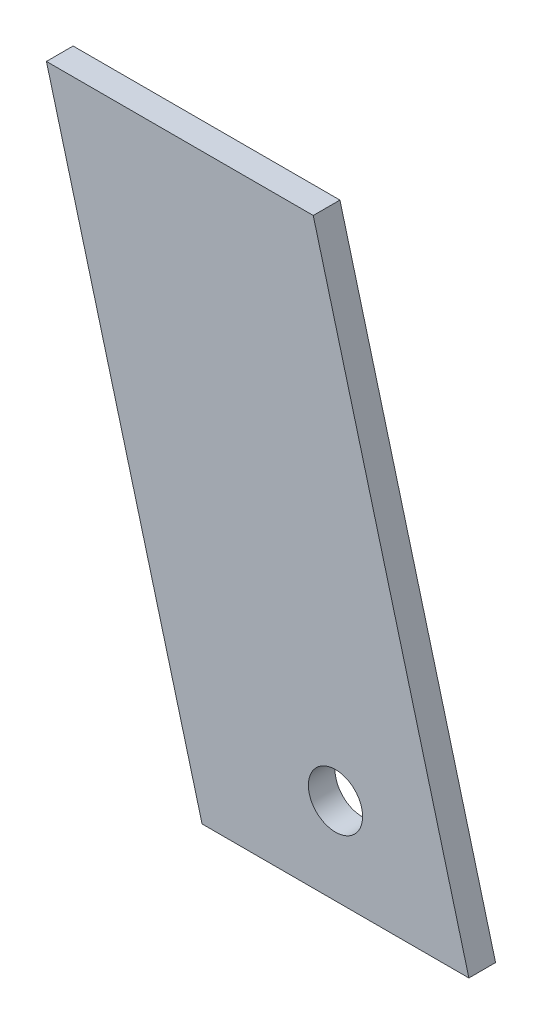
SolidWorks part; units mm, degrees
ref_plane "前视基准面" through (0, 0, 0) normal (0, 0, 1) x (1, 0, 0)
ref_plane "上视基准面" through (0, 0, 0) normal (0, 1, 0) x (1, 0, 0)
ref_plane "右视基准面" through (0, 0, 0) normal (1, 0, 0) x (0, 0, -1)
other "Configuration Table"
sketch "草图1" plane through (0, 0, 0) normal (0, 0, 1) x (1, 0, 0)
  line L0 (-30, -36) -> (30, -36)
  line L1 (30, -36) -> (65, -167)
  line L2 (65, -167) -> (5, -167)
  line L3 (5, -167) -> (-30, -36)
  point P0 (0, 0)
  dimension "D1" = 30
  dimension "D2" = 35
  dimension "D3" = 60
  dimension "D4" = 95
  dimension "D5" = 131
  dimension "D6" = 167
extrude "凸台-拉伸1" add sketch "草图1" against normal mid plane 6
sketch "草图2" plane through (0, 0, 0) normal (0, 0, 1) x (1, 0, 0)
  circle A0 centre (35, -147.5) radius 6.1
  point P0 (0, 0)
  dimension "D1" = 12.2
  dimension "D2" = 35
  dimension "D3" = 147.5
extrude "切除-拉伸1" cut sketch "草图2" against normal mid plane 30
